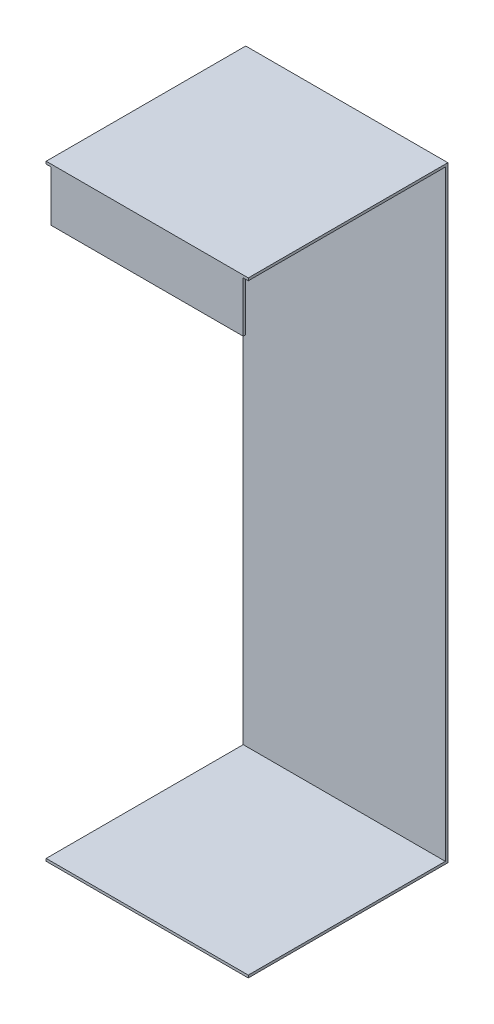
SolidWorks part; units mm, degrees
ref_plane "Front Plane" through (0, 0, 0) normal (0, 0, 1) x (1, 0, 0)
ref_plane "Top Plane" through (0, 0, 0) normal (0, 1, 0) x (1, 0, 0)
ref_plane "Right Plane" through (0, 0, 0) normal (1, 0, 0) x (0, 0, -1)
sketch "Sketch1" plane through (0, 0, 0) normal (0, 0, 1) x (1, 0, 0)
  line L1 (-40, 120) -> (40, 120)
  line L2 (-40, 120) -> (-40, -120)
  line L3 (-40, -120) -> (40, -120)
  line L4 (40, 120) -> (40, -120)
  line L5 (-40, 120) -> (40, -120) construction
  line L6 (-40, -120) -> (40, 120) construction
  point P0 (0, 0)
  dimension "D1" = 80
  dimension "D2" = 240
extrude "Boss-Extrude1" add sketch "Sketch1" along normal blind 1
sketch "Sketch2" plane through (0, 0, 1) normal (0, 0, 1) x (1, 0, 0)
  line L0 (40, -120) -> (40, 120) construction
  line L1 (-40, 120) -> (40, 120)
  line L2 (-40, 120) -> (-40, 119)
  line L3 (-40, 119) -> (40, 119)
  line L4 (40, 120) -> (40, 119)
  line L6 (-40, -120) -> (40, -120)
  line L7 (-40, -120) -> (-40, -119)
  line L8 (-40, -119) -> (40, -119)
  line L9 (40, -120) -> (40, -119)
  dimension "D1" = 1
  dimension "D2" = 1
extrude "Boss-Extrude2" add sketch "Sketch2" along normal blind 78
sketch "Sketch3" plane through (0, 0, 79) normal (0, 0, 1) x (1, 0, 0)
  line L1 (-40, 119) -> (40, 119)
  line L2 (-40, 119) -> (-40, 99)
  line L3 (-40, 99) -> (40, 99)
  line L4 (40, 119) -> (40, 99)
  dimension "D1" = 20
extrude "Boss-Extrude3" add sketch "Sketch3" against normal blind 1
sketch "Sketch4" plane through (0, 99, 0) normal (0, 1, 0) x (1, 0, 0)
  line L0 (0, -79) -> (0, -59.4972) construction
  line L1 (-40, -79) -> (-38, -79)
  line L2 (-40, -79) -> (-40, -78)
  line L3 (-40, -78) -> (-38, -78)
  line L4 (-38, -79) -> (-38, -78)
  line L5 (40, -79) -> (-40, -79) construction
  line L6 (38, -79) -> (38, -78)
  line L7 (40, -78) -> (38, -78)
  line L8 (40, -79) -> (40, -78)
  line L9 (40, -79) -> (38, -79)
  dimension "D1" = 1
  dimension "D2" = 2
extrude "Cut-Extrude1" cut sketch "Sketch4" along normal up to surface (20 mm away) up to face at (0, 119, 39.5)
